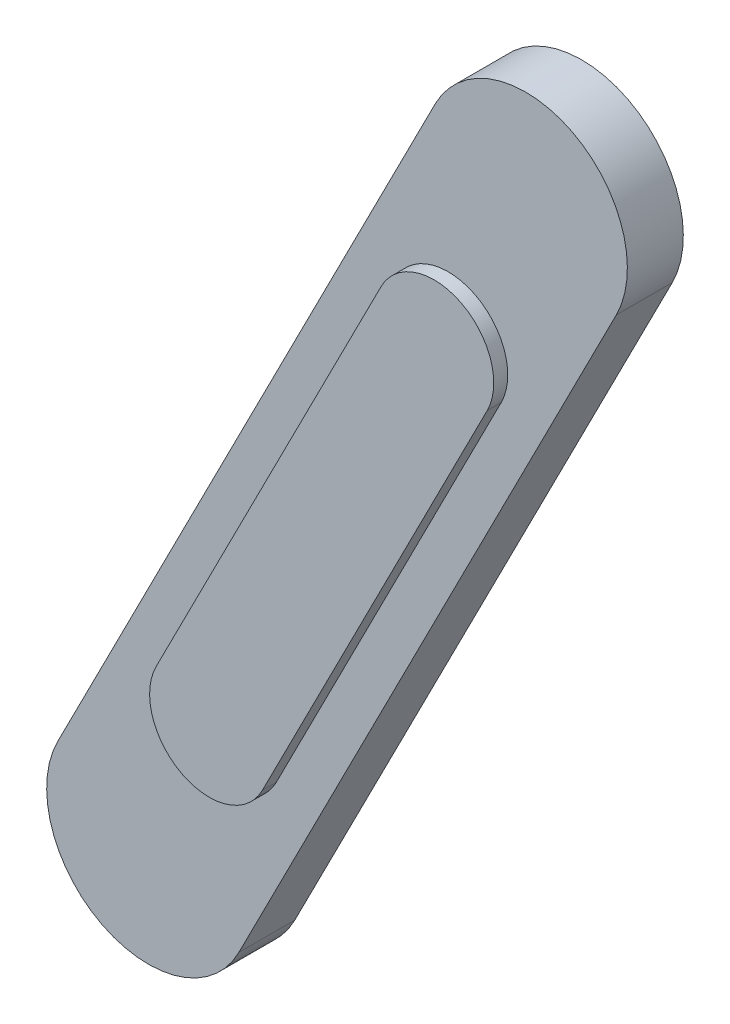
SolidWorks part; units mm, degrees
ref_plane "Front Plane" through (0, 0, 0) normal (0, 0, 1) x (1, 0, 0)
ref_plane "Top Plane" through (0, 0, 0) normal (0, 1, 0) x (1, 0, 0)
ref_plane "Right Plane" through (0, 0, 0) normal (1, 0, 0) x (0, 0, -1)
sketch "Sketch2" plane through (0, 0, 0) normal (0, 0, 1) x (1, 0, 0)
  line L0 (0, 7.8572) -> (14.351, 36.0221)
  line L1 (0.8578, 9.5406) -> (14.351, 36.0221) construction
  line L2 (-2.3789, 11.1898) -> (11.1144, 37.6713)
  line L3 (4.0944, 7.8914) -> (17.5877, 34.3729)
  arc A0 (-2.3789, 11.1898) -> (4.0944, 7.8914) centre (0.8578, 9.5406) ccw
  arc A1 (17.5877, 34.3729) -> (11.1144, 37.6713) centre (14.351, 36.0221) ccw
  circle A2 centre (0.8578, 9.5406) radius 1.5
  circle A3 centre (14.351, 36.0221) radius 1.5
  point P3 (7.6044, 22.7813)
  dimension "D1" = 3
  dimension "D2" = 3
extrude "Boss-Extrude1" add sketch "Sketch2" along normal mid plane 2
sketch "Sketch3" plane through (0, 0, 1) normal (0, 0, 1) x (1, 0, 0)
  line L0 (3.5361, 14.797) -> (11.5754, 30.5748) construction
  line L1 (1.6374, 15.7644) -> (9.6768, 31.5422)
  line L2 (5.4348, 13.8295) -> (13.4741, 29.6073)
  line L3 (4.0944, 7.8914) -> (17.5877, 34.3729) construction
  line L4 (0.8578, 9.5406) -> (14.351, 36.0221) construction
  arc A0 (1.6374, 15.7644) -> (5.4348, 13.8295) centre (3.5361, 14.797) ccw
  arc A1 (13.4741, 29.6073) -> (9.6768, 31.5422) centre (11.5754, 30.5748) ccw
  circle A2 centre (0.8578, 9.5406) radius 1.5 construction
  point P2 (7.5558, 22.6859)
extrude "Boss-Extrude2" add sketch "Sketch3" along normal mid plane 1
sketch "Sketch4" plane through (0, 0, 1) normal (0, 0, 1) x (1, 0, 0)
  circle A0 centre (0.8578, 9.5406) radius 1.5 construction
  circle A1 centre (0.8578, 9.5406) radius 1.5
extrude "Boss-Extrude3" add sketch "Sketch4" against normal blind 0.1
sketch "Sketch5" plane through (0, 0, 1) normal (0, 0, 1) x (1, 0, 0)
  circle A0 centre (14.351, 36.0221) radius 1.5 construction
  circle A1 centre (14.351, 36.0221) radius 1.5
extrude "Boss-Extrude5" add sketch "Sketch5" against normal blind 0.1
